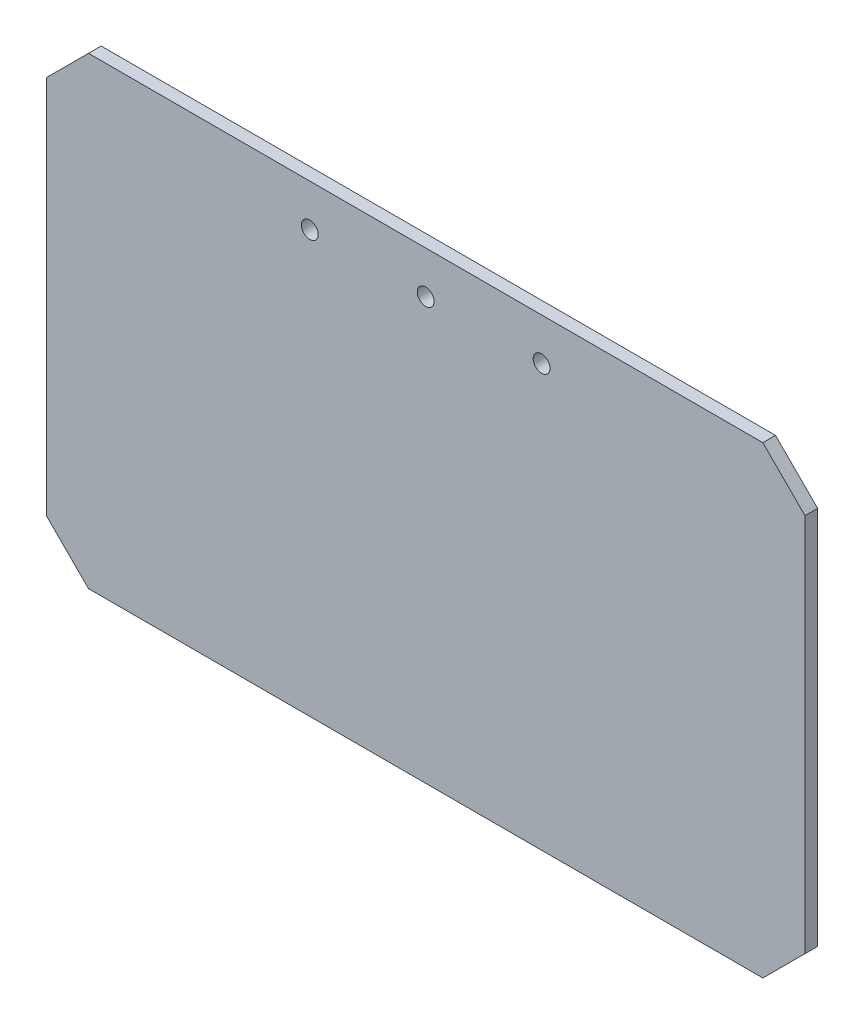
from build123d import *

# Parameters (mm, degrees)
SKETCH1_R           = 2
BOSS_EXTRUDE1_DEPTH = 3


with BuildPart() as part:
    # Sketch1 → Boss-Extrude1 (new body)
    with BuildSketch(Plane.XY):
        Polygon((10, 0), (170, 0), (180, -10), (180, -100), (170, -110), (10, -110), (0, -100), (0, -10), align=None)
        with Locations((90, -10)):
            Circle(SKETCH1_R, mode=Mode.SUBTRACT)
        with Locations((117.5, -10)):
            Circle(SKETCH1_R, mode=Mode.SUBTRACT)
        with Locations((62.5, -10)):
            Circle(SKETCH1_R, mode=Mode.SUBTRACT)
    extrude(amount=BOSS_EXTRUDE1_DEPTH)


solid = part.part
